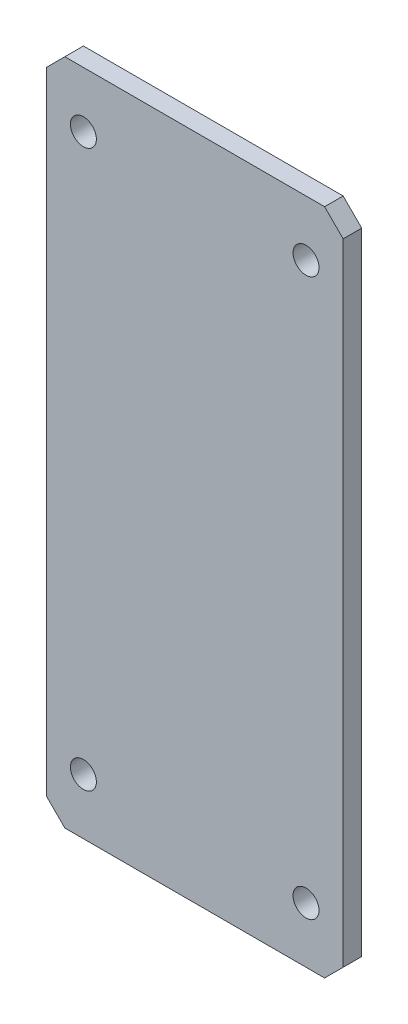
from build123d import *

# Parameters (mm, degrees)
SKETCH_1_W          = 80
SKETCH_1_H          = 180
EXTRUDE_1_DEPTH     = 5
CHAMFER_1_SIZE      = 5
SKETCH_2_R          = 3.5
CUT_EXTRUDE_1_DEPTH = 5


with BuildPart() as part:
    # 草图1 → 凸台-拉伸1 (new body)
    with BuildSketch(Plane.XY):
        Rectangle(SKETCH_1_W, SKETCH_1_H)
    extrude(amount=EXTRUDE_1_DEPTH)

    # 倒角1
    chamfer_1_edges = [part.edges().sort_by_distance(p)[0] for p in [
        (40, -90, 2.5),
        (-40, -90, 2.5),
        (-40, 90, 2.5),
        (40, 90, 2.5),
    ]]
    chamfer(chamfer_1_edges, length=CHAMFER_1_SIZE)

    # 草图2 → 切除-拉伸1 (cut)
    with BuildSketch(Plane.XY.offset(5)):
        with Locations((-30, 75)):
            Circle(SKETCH_2_R)
        with Locations((30, 75)):
            Circle(SKETCH_2_R)
        with Locations((-30, -75)):
            Circle(SKETCH_2_R)
        with Locations((30, -75)):
            Circle(SKETCH_2_R)
    extrude(amount=-CUT_EXTRUDE_1_DEPTH, mode=Mode.SUBTRACT)


solid = part.part
